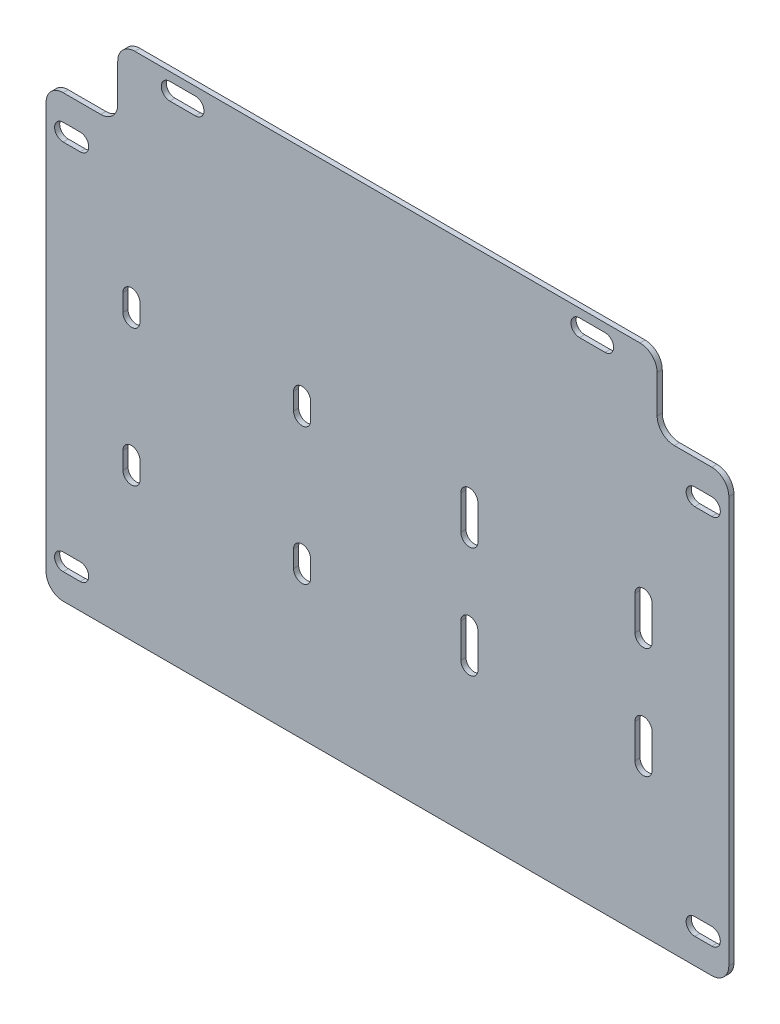
from build123d import *

# Parameters (mm, degrees)
SKETCH1_W           = 400
SKETCH1_H           = 342
BOSS_EXTRUDE1_DEPTH = 3
SKETCH3_W           = 86.448848967
SKETCH3_H           = 526.142419803
CUT_EXTRUDE2_DEPTH  = 527.282243668
FILLET1_R           = 10
CUT_EXTRUDE3_DEPTH  = 527.282243668
SKETCH5_W           = 336
SKETCH5_H           = 215.570811559
CUT_EXTRUDE4_DEPTH  = 10


with BuildPart() as part:
    # Sketch1 → Boss-Extrude1 (new body)
    with BuildSketch(Plane.XY):
        with Locations((200, -171)):
            Rectangle(SKETCH1_W, SKETCH1_H)
        with BuildLine():
            Line((253, -128.5), (253, -148.5))
            ThreePointArc((253, -148.5), (248, -153.5), (243, -148.5))
            Line((243, -148.5), (243, -128.5))
            ThreePointArc((243, -128.5), (248, -123.5), (253, -128.5))
        make_face(mode=Mode.SUBTRACT)
        with BuildLine():
            Line((345, -128.5), (345, -148.5))
            ThreePointArc((345, -148.5), (350, -153.5), (355, -148.5))
            Line((355, -148.5), (355, -128.5))
            ThreePointArc((355, -128.5), (350, -123.5), (345, -128.5))
        make_face(mode=Mode.SUBTRACT)
        with BuildLine():
            Line((345, -213.5), (345, -193.5))
            ThreePointArc((345, -193.5), (350, -188.5), (355, -193.5))
            Line((355, -193.5), (355, -213.5))
            ThreePointArc((355, -213.5), (350, -218.5), (345, -213.5))
        make_face(mode=Mode.SUBTRACT)
        with BuildLine():
            Line((253, -213.5), (253, -193.5))
            ThreePointArc((253, -193.5), (248, -188.5), (243, -193.5))
            Line((243, -193.5), (243, -213.5))
            ThreePointArc((243, -213.5), (248, -218.5), (253, -213.5))
        make_face(mode=Mode.SUBTRACT)
        with BuildLine():
            Line((72.5, -5), (87.5, -5))
            ThreePointArc((87.5, -5), (92.5, -10), (87.5, -15))
            Line((87.5, -15), (72.5, -15))
            ThreePointArc((72.5, -15), (67.5, -10), (72.5, -5))
        make_face(mode=Mode.SUBTRACT)
        with BuildLine():
            Line((327.5, -5), (312.5, -5))
            ThreePointArc((312.5, -5), (307.5, -10), (312.5, -15))
            Line((312.5, -15), (327.5, -15))
            ThreePointArc((327.5, -15), (332.5, -10), (327.5, -5))
        make_face(mode=Mode.SUBTRACT)
        with BuildLine():
            Line((327.5, -337), (312.5, -337))
            ThreePointArc((312.5, -337), (307.5, -332), (312.5, -327))
            Line((312.5, -327), (327.5, -327))
            ThreePointArc((327.5, -327), (332.5, -332), (327.5, -337))
        make_face(mode=Mode.SUBTRACT)
        with BuildLine():
            Line((72.5, -337), (87.5, -337))
            ThreePointArc((87.5, -337), (92.5, -332), (87.5, -327))
            Line((87.5, -327), (72.5, -327))
            ThreePointArc((72.5, -327), (67.5, -332), (72.5, -337))
        make_face(mode=Mode.SUBTRACT)
        with BuildLine():
            Line((55, -126), (55, -136))
            ThreePointArc((55, -136), (50, -141), (45, -136))
            Line((45, -136), (45, -126))
            ThreePointArc((45, -126), (50, -121), (55, -126))
        make_face(mode=Mode.SUBTRACT)
        with BuildLine():
            Line((155, -126), (155, -136))
            ThreePointArc((155, -136), (150, -141), (145, -136))
            Line((145, -136), (145, -126))
            ThreePointArc((145, -126), (150, -121), (155, -126))
        make_face(mode=Mode.SUBTRACT)
        with BuildLine():
            Line((155, -216), (155, -206))
            ThreePointArc((155, -206), (150, -201), (145, -206))
            Line((145, -206), (145, -216))
            ThreePointArc((145, -216), (150, -221), (155, -216))
        make_face(mode=Mode.SUBTRACT)
        with BuildLine():
            Line((55, -216), (55, -206))
            ThreePointArc((55, -206), (50, -201), (45, -206))
            Line((45, -206), (45, -216))
            ThreePointArc((45, -216), (50, -221), (55, -216))
        make_face(mode=Mode.SUBTRACT)
    extrude(amount=BOSS_EXTRUDE1_DEPTH)

    # Sketch3 → Cut-Extrude2 (cut, through all)
    with BuildSketch(Plane.XY.offset(3)):
        with Locations((-1.224424484, -563.071209901)):
            Rectangle(SKETCH3_W, SKETCH3_H)
        with Locations((401.224424484, -563.071209901)):
            Rectangle(SKETCH3_W, SKETCH3_H)
        with Locations((401.224424484, 221.071209902)):
            Rectangle(SKETCH3_W, SKETCH3_H)
        with Locations((-1.224424484, 221.071209902)):
            Rectangle(SKETCH3_W, SKETCH3_H)
    extrude(amount=-CUT_EXTRUDE2_DEPTH, mode=Mode.SUBTRACT)

    # Fillet1
    fillet1_edges = [part.edges().sort_by_distance(p)[0] for p in [
        (358, 0, 1.5),
        (42, 0, 1.5),
        (400, -300, 1.5),
        (400, -42, 1.5),
        (42, -342, 1.5),
        (358, -342, 1.5),
        (0, -300, 1.5),
        (0, -42, 1.5),
        (42, -42, 1.5),
        (358, -42, 1.5),
        (358, -300, 1.5),
        (42, -300, 1.5),
    ]]
    fillet(fillet1_edges, radius=FILLET1_R)

    # Sketch4 → Cut-Extrude3 (cut, through all)
    with BuildSketch(Plane.XY.offset(3)):
        with BuildLine():
            Line((10, -57), (20, -57))
            ThreePointArc((20, -57), (25, -62), (20, -67))
            Line((20, -67), (10, -67))
            ThreePointArc((10, -67), (5, -62), (10, -57))
        make_face()
        with BuildLine():
            Line((390, -57), (380, -57))
            ThreePointArc((380, -57), (375, -62), (380, -67))
            Line((380, -67), (390, -67))
            ThreePointArc((390, -67), (395, -62), (390, -57))
        make_face()
        with BuildLine():
            Line((390, -285), (380, -285))
            ThreePointArc((380, -285), (375, -280), (380, -275))
            Line((380, -275), (390, -275))
            ThreePointArc((390, -275), (395, -280), (390, -285))
        make_face()
        with BuildLine():
            Line((10, -285), (20, -285))
            ThreePointArc((20, -285), (25, -280), (20, -275))
            Line((20, -275), (10, -275))
            ThreePointArc((10, -275), (5, -280), (10, -285))
        make_face()
    extrude(amount=-CUT_EXTRUDE3_DEPTH, mode=Mode.SUBTRACT)

    # Sketch5 → Cut-Extrude4 (cut)
    with BuildSketch(Plane.XY.offset(3)):
        with Locations((200, -407.78540578)):
            Rectangle(SKETCH5_W, SKETCH5_H)
    extrude(amount=-CUT_EXTRUDE4_DEPTH, mode=Mode.SUBTRACT)


solid = part.part
